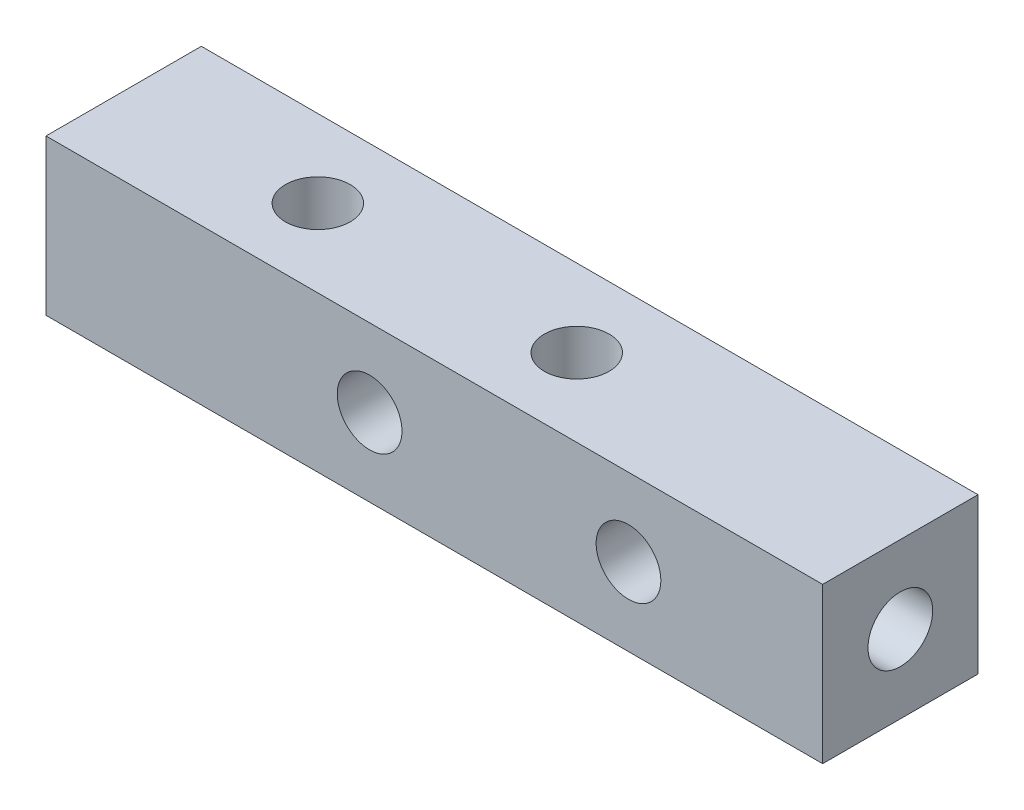
from build123d import *

# Parameters (mm, degrees)
SKETCH_1_W             = 30
SKETCH_1_H             = 6
EXTRUDE_1_DEPTH        = 6
HOLE_WIZARD_M3_1_D     = 2.5
HOLE_WIZARD_M3_2_D     = 2.5
HOLE_WIZARD_M3_3_D     = 2.5
HOLE_WIZARD_M3_3_DEPTH = 4.248924226
HOLE_WIZARD_M3_3_TIP   = 0.751075774
HOLE_WIZARD_M3_4_D     = 2.5
HOLE_WIZARD_M3_4_DEPTH = 4.248924226
HOLE_WIZARD_M3_4_TIP   = 0.751075774


with BuildPart() as part:
    # 草图1 → 凸台-拉伸1 (new body)
    with BuildSketch(Plane(origin=(0, 0, 0), x_dir=(1, 0, 0), z_dir=(0, 1, 0))):
        Rectangle(SKETCH_1_W, SKETCH_1_H)
    extrude(amount=EXTRUDE_1_DEPTH)

    # M3 螺纹孔1 (through all)
    with Locations(Plane.XY.offset(3)):
        with Locations((-2.5, 3), (7.5, 3)):
            Hole(HOLE_WIZARD_M3_1_D / 2)

    # M3 螺纹孔2 (through all)
    with Locations(Plane(origin=(0, 6, 0), x_dir=(1, 0, 0), z_dir=(0, 1, 0))):
        with Locations((2.5, 0), (-7.5, 0)):
            Hole(HOLE_WIZARD_M3_2_D / 2)

    # M3 螺纹孔3
    with Locations(Plane.ZY.offset(15)):
        with Locations((0, 3)):
            Hole(HOLE_WIZARD_M3_3_D / 2, depth=HOLE_WIZARD_M3_3_DEPTH)
            with Locations((0, 0, -(HOLE_WIZARD_M3_3_DEPTH + HOLE_WIZARD_M3_3_TIP / 2))):  # 118° drill point
                Cone(0, HOLE_WIZARD_M3_3_D / 2, HOLE_WIZARD_M3_3_TIP, mode=Mode.SUBTRACT)

    # M3 螺纹孔4
    with Locations(Plane(origin=(15, 0, 0), x_dir=(0, 0, -1), z_dir=(1, 0, 0))):
        with Locations((0, 3)):
            Hole(HOLE_WIZARD_M3_4_D / 2, depth=HOLE_WIZARD_M3_4_DEPTH)
            with Locations((0, 0, -(HOLE_WIZARD_M3_4_DEPTH + HOLE_WIZARD_M3_4_TIP / 2))):  # 118° drill point
                Cone(0, HOLE_WIZARD_M3_4_D / 2, HOLE_WIZARD_M3_4_TIP, mode=Mode.SUBTRACT)


solid = part.part
